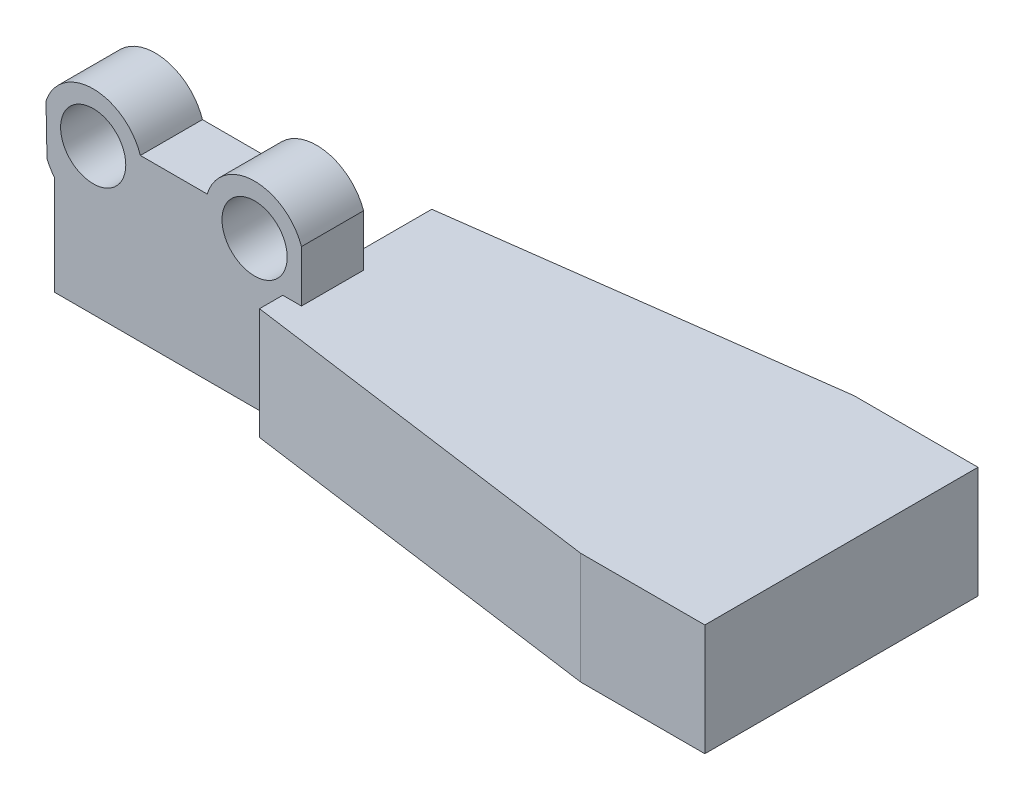
SolidWorks part; units mm, degrees
ref_plane "Front Plane" through (0, 0, 0) normal (0, 0, 1) x (1, 0, 0)
ref_plane "Top Plane" through (0, 0, 0) normal (0, 1, 0) x (1, 0, 0)
ref_plane "Right Plane" through (0, 0, 0) normal (1, 0, 0) x (0, 0, -1)
other "Configuration Table"
sketch "Sketch1" plane through (0, 0, 0) normal (0, 0, 1) x (1, 0, 0)
  line L0 (10, -2.4993) -> (39.9926, -4.0155)
  line L1 (0, 0) -> (10, 0)
  line L2 (0, 0) -> (0, -5)
  line L3 (0, -5) -> (10, -5)
  line L4 (10, 0) -> (10, -2.4993)
  line L5 (10, -5) -> (39.9926, -5)
  line L6 (39.9926, -5) -> (39.9926, -4.0155)
  line L7 (10, -2.4993) -> (10, -5)
  dimension "D1" = 10
  dimension "D2" = 5
extrude "Boss-Extrude1" add sketch "Sketch1" along normal blind 20 contours L1 L4 L0 L6 L5 L3 L2
sketch "Sketch2" plane through (0, 0, 0) normal (0, 1, 0) x (1, 0, 0)
  line L0 (0, 0) -> (0, -5) construction
  line L1 (0, -20) -> (0, 0) construction
  line L2 (0, -5) -> (39.9926, -20)
  line L3 (39.9926, -20) -> (0, -20)
  line L4 (0, -20) -> (0, -5)
extrude "Cut-Extrude1" cut sketch "Sketch2" against normal blind 20
sketch "Sketch3" plane through (0, 0, 0) normal (0, 0, -1) x (-1, 0, 0)
  line L0 (-10, -2.4993) -> (0, -2.5) construction
  line L1 (-10, 0) -> (-10, -2.4993) construction
  line L2 (0, 0) -> (0, -5) construction
  circle A1 centre (-7.7289, -2.4995) radius 2
extrude "Cut-Extrude2" cut sketch "Sketch3" against normal blind 20
sketch "Sketch4" plane through (0, 0, 0) normal (0, 1, 0) x (1, 0, 0)
  line L0 (0, -5) -> (10, -5)
  line L1 (10, -8.7507) -> (10, 0) construction
  line L2 (10, -5) -> (10, -8.7507)
  line L3 (10, -8.7507) -> (0, -5)
extrude "Cut-Extrude3" cut sketch "Sketch4" against normal blind 20
sketch "Sketch5" plane through (0, 0, 5) normal (0, 0, 1) x (1, 0, 0)
  line L0 (0, -2.5) -> (10, -2.4993) construction
  line L1 (0, -5) -> (0, 0) construction
  circle A0 centre (1.5846, -2.4999) radius 1
sketch "Sketch6" plane through (0, 0, 0) normal (-1, 0, 0) x (0, 0, 1)
  line L1 (0, 0) -> (5, 0)
  line L2 (0, 0) -> (0, -5)
  line L3 (0, -5) -> (5, -5)
  line L4 (5, 0) -> (5, -5)
extrude "Boss-Extrude3" add sketch "Sketch6" along normal blind 5
fillet "Fillet1" radius 2 2 edges at (10, -2.4993, 6.8753) (10, -2.4993, 2.5)
sketch "Sketch9" plane through (10, 0, 0) normal (-1, 0, 0) x (0, 0, 1)
  line L0 (5, -3.4999) -> (5, -1.4999) construction
  line L1 (10.3077, -0.3833) -> (5, -0.3833)
  line L2 (10.3077, -0.3833) -> (10.3077, -2.4999)
  line L3 (10.3077, -2.4999) -> (5, -2.4999)
  line L4 (5, -0.3833) -> (5, -2.4999)
extrude "Cut-Extrude5" cut sketch "Sketch9" against normal blind 5
sketch "Sketch10" plane through (39.9926, 0, 0) normal (1, 0, 0) x (0, 0, -1)
  line L1 (-20, -4.0155) -> (0, -4.0155)
  line L2 (-20, -4.0155) -> (-20, -5)
  line L3 (-20, -5) -> (0, -5)
  line L4 (0, -4.0155) -> (0, -5)
extrude "Boss-Extrude5" add sketch "Sketch10" along normal blind 10
sketch "Sketch12" plane through (-5, 0, 0) normal (-1, 0, 0) x (0, 0, 1)
  line L1 (0, 0) -> (5, 0)
  line L2 (0, 0) -> (0, -5)
  line L3 (0, -5) -> (5, -5)
  line L4 (5, 0) -> (5, -5)
extrude "Boss-Extrude6" add sketch "Sketch12" along normal blind 5
sketch "Sketch14" plane through (0, 0, 5) normal (0, 0, 1) x (1, 0, 0)
  line L0 (7.7289, -2.4995) -> (-5.2711, -2.4995) construction
  circle A0 centre (-5.2711, -2.4995) radius 2.5
extrude "Boss-Extrude8" add sketch "Sketch14" along normal blind 8
sketch "Sketch15" plane through (0, 0, 5) normal (0, 0, 1) x (1, 0, 0)
  line L0 (10, -5) -> (-10, -5) construction
  line L1 (-10, 0) -> (-8, 0)
  line L2 (-10, 0) -> (-10, -5)
  line L3 (-10, -5) -> (-8, -5)
  line L4 (-8, 0) -> (-8, -5)
extrude "Cut-Extrude6" cut sketch "Sketch15" against normal through all
fillet "Fillet2" radius 0.5 2 edges at (10, 0, 2.5)
fillet "Fillet3" radius 2 1 edges at (-8, 0, 2.5)
fillet "Fillet4" radius 2 1 edges at (-8, -5, 2.5)
sketch "Sketch17" plane through (0, 0, 13) normal (0, 0, 1) x (1, 0, 0)
  line L0 (-5.2711, -2.4995) -> (-5.2711, 0.0005) construction
  circle A0 centre (-5.2711, -2.4995) radius 2.5 construction
ref_plane "Plane1" through (-5.2711, 0, 0) normal (1, 0, 0) x (0, 1, 0)
sketch "Sketch19" plane through (-5.2711, 0, 1.9984) normal (1, 0, 0) x (0, 1, 0)
  line L3 (0.0006, 9) -> (-0.9994, 9)
  line L4 (-0.9994, 9) -> (-0.9994, 7.9999)
  line L5 (-0.9994, 7.9999) -> (0.0006, 7.9999)
  line L6 (0.0006, 7.9999) -> (0.0006, 9)
  line L7 (-2.4993, 13) -> (-2.4999, 5) construction
  line L9 (-4, 8.0001) -> (-5, 8.0002)
  line L10 (-5, 8.0002) -> (-4.9999, 9.0003)
  line L11 (-4.9999, 9.0003) -> (-3.9999, 9.0002)
  line L12 (-3.9999, 9.0002) -> (-4, 8.0001)
revolve "Cut-Revolve1" cut sketch "Sketch19" angle 46 about L7
sketch "Sketch20" plane through (0, 0, 5) normal (0, 0, 1) x (1, 0, 0)
  circle A0 centre (7.7289, -2.4995) radius 4
extrude "Boss-Extrude9" add sketch "Sketch20" against normal through all
sketch "Sketch21" plane through (0, 0, 5) normal (0, 0, 1) x (1, 0, 0)
  circle A0 centre (7.7289, -2.4995) radius 2.625
sketch "Sketch23" plane through (0, 0, 5) normal (0, 0, 1) x (1, 0, 0)
  line L0 (0, -2.5) -> (10, -2.4993) construction
  line L1 (8.9411, -2.4994) -> (35.3949, -2.4994)
  line L2 (8.9411, -2.4994) -> (8.9411, -3.3189)
  line L3 (8.9411, -3.3189) -> (35.3949, -3.3189)
  line L4 (35.3949, -2.4994) -> (35.3949, -3.3189)
extrude "Cut-Extrude8" cut sketch "Sketch23" along normal through all
sketch "Sketch24" plane through (0, 0, 0) normal (0, 0, -1) x (-1, 0, 0)
  circle A0 centre (5.2711, -2.4995) radius 4
extrude "Boss-Extrude10" add sketch "Sketch24" against normal blind 5
sketch "Sketch25" plane through (0, 0, 0) normal (0, 0, -1) x (-1, 0, 0)
  circle A0 centre (5.2711, -2.4995) radius 2.625
sketch "Sketch26" plane through (0, 0, 13) normal (0, 0, 1) x (1, 0, 0)
  circle A0 centre (-5.2711, -2.4995) radius 10.8429
extrude "Cut-Extrude9" cut sketch "Sketch26" against normal blind 8
sketch "Sketch27" plane through (0, 0, 5) normal (0, 0, 1) x (1, 0, 0)
  line L0 (-5.2711, -2.4995) -> (-5.2711, 0.0005) construction
  line L1 (7.7289, -2.4995) -> (7.7289, 0.1255) construction
  circle A0 centre (-5.2711, -1.2495) radius 2.625
  circle A1 centre (7.7289, -2.4995) radius 2.625 construction
  circle A2 centre (7.7289, -1.187) radius 2.625
sketch "Sketch28" plane through (0, 0, 0) normal (0, 0, -1) x (-1, 0, 0)
  circle A0 centre (-7.7289, -1.187) radius 4
  circle A1 centre (5.2711, -1.2495) radius 4
extrude "Boss-Extrude11" add sketch "Sketch28" against normal blind 5
sketch "Sketch29" plane through (0, 0, 0) normal (0, 0, -1) x (-1, 0, 0)
  line L0 (-10.851, -5) -> (9.678, -5)
  line L1 (9.678, -5) -> (5.4495, -9.2285)
  line L2 (5.4495, -9.2285) -> (-11.8183, -9.821)
  line L3 (-11.8183, -9.821) -> (-12.0426, -7.5304)
  line L4 (-12.0426, -7.5304) -> (-10.851, -5)
extrude "Cut-Extrude10" cut sketch "Sketch29" against normal blind 5
sketch "Sketch30" plane through (0, 0, 0) normal (0, 0, -1) x (-1, 0, 0)
  line L0 (-11.7281, -2.5793) -> (-11.5054, -2.5793)
  line L1 (-11.5054, -2.5793) -> (-11.5054, 0.7603)
  line L2 (-11.5054, 0.7603) -> (-9.1187, 5.5657)
  line L3 (-9.1187, 5.5657) -> (0.4121, 5.3735)
  line L4 (0.4121, 5.3735) -> (6.0024, 5.3735)
  line L5 (6.0024, 5.3735) -> (8.0527, 3.8037)
  line L6 (8.0527, 3.8037) -> (9.0709, 0)
  line L7 (9.0709, 0) -> (8.9908, -3.9703)
  line L8 (8.9908, -3.9703) -> (10.2632, -3.1962)
  line L9 (10.2632, -3.1962) -> (9.8627, 1.0326)
  line L10 (9.8627, 1.0326) -> (8.0527, 6.1584)
  line L11 (8.0527, 6.1584) -> (0.8125, 7.3598)
  line L12 (0.8125, 7.3598) -> (-5.4666, 6.9593)
  line L13 (-5.4666, 6.9593) -> (-11.9307, 6.3472)
  line L14 (-11.9307, 6.3472) -> (-14.3685, 3.163)
  line L15 (-14.3685, 3.163) -> (-14.5975, 0.4773)
  line L16 (-14.5975, 0.4773) -> (-13.7279, -1.9852)
  line L17 (-13.7279, -1.9852) -> (-11.7281, -2.5793)
  arc A0 (9.2219, -1.8745) -> (1.4712, 0) centre (5.2711, -1.2495) ccw construction
  arc A1 (8.3932, -5) -> (9.2219, -1.8745) centre (5.2711, -2.4995) ccw construction
extrude "Cut-Extrude11" cut sketch "Sketch30" against normal blind 5
extrude "Cut-Extrude12" cut sketch "Sketch27" against normal blind 5
sketch "Sketch31" plane through (0, -5, 0) normal (0, -1, 0) x (1, 0, 0)
  line L0 (-8.3932, 0) -> (49.9926, 0)
  line L1 (49.9926, 0) -> (49.9926, 20)
  line L2 (49.9926, 20) -> (39.9926, 20)
  line L3 (39.9926, 20) -> (10, 8.7507)
  line L5 (10, 8.7507) -> (10, 5)
  line L6 (10, 8.7507) -> (10, 5) construction
  line L7 (10, 5) -> (-8.3932, 5)
  line L8 (-8.3932, 5) -> (-8.3932, 0)
extrude "Boss-Extrude12" add sketch "Sketch31" along normal blind 8
sketch "Sketch33" plane through (0, -4.0155, 0) normal (0, 1, 0) x (1, 0, 0)
  line L1 (39.9926, -20) -> (11.5054, -20)
  line L2 (39.9926, -20) -> (39.9926, 0)
  line L3 (39.9926, 0) -> (11.5054, 0)
  line L4 (11.5054, -20) -> (11.5054, 0)
extrude "Cut-Extrude13" cut sketch "Sketch33" along normal through all
sketch "Sketch34" plane through (0, -3.3189, 0) normal (0, 1, 0) x (1, 0, 0)
  line L0 (10, -5) -> (11.5054, -5)
  line L1 (11.5054, -5) -> (11.5054, -9.3153)
  line L2 (11.5054, -9.3153) -> (10, -8.7507)
  line L3 (10, -8.7507) -> (10, -5)
extrude "Cut-Extrude14" cut sketch "Sketch34" against normal up to surface (0.6966 mm away)
sketch "Sketch35" plane through (0, -13, 0) normal (0, -1, 0) x (1, 0, 0)
  line L0 (10, 6.8753) -> (39.9926, 11)
  line L1 (39.9926, 11) -> (49.9926, 11)
  line L2 (49.9926, 0) -> (49.9926, 20) construction
  line L3 (49.9926, 11) -> (49.9926, 20)
  line L4 (49.9926, 20) -> (39.9926, 20)
  line L6 (10, 8.7507) -> (10, 5) construction
  line L7 (39.9926, 20) -> (10, 8.7507)
  line L8 (10, 8.7507) -> (10, 6.8753)
  dimension "D1" = 11
extrude "Cut-Extrude15" cut sketch "Sketch35" against normal blind 10
sketch "Sketch36" plane through (0, -4.0155, 0) normal (0, 1, 0) x (1, 0, 0)
  line L0 (49.9926, 0) -> (49.9926, 11)
  line L1 (49.9926, 0) -> (49.9926, -11) construction
  line L2 (49.9926, 11) -> (39.9926, 11)
  line L3 (39.9926, 11) -> (10, 7)
  line L4 (10, 7) -> (10, 0)
  line L5 (11.5054, 0) -> (3.9091, 0) construction
  line L6 (10, -5) -> (10, -6.8753) construction
  line L7 (49.9926, 0) -> (10, 0)
  dimension "D1" = 11
  dimension "D2" = 7
extrude "Boss-Extrude13" add sketch "Sketch36" against normal up to surface (8.9845 mm away)
